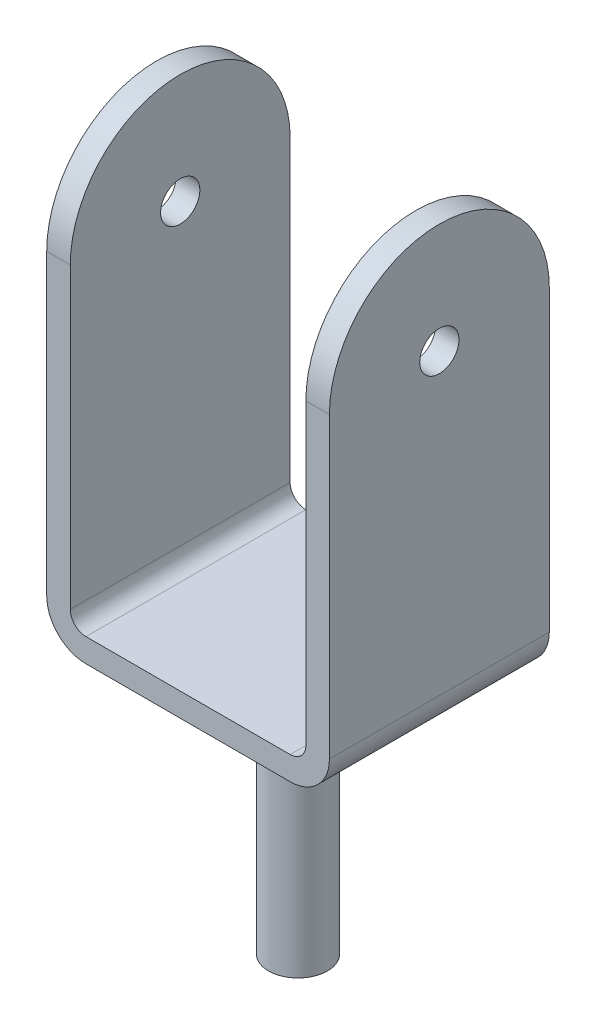
from build123d import *
from build123d.topology import SkipClean

# Parameters (mm, degrees)
BOSS_EXTRUDE1_DEPTH = 280
FILLET1_R           = 50
BOSS_EXTRUDE3_START = -30
BOSS_EXTRUDE3_DEPTH = 30
CUT_EXTRUDE5_START  = -30
CUT_EXTRUDE5_DEPTH  = 30
BOSS_EXTRUDE4_DEPTH = 30
CUT_EXTRUDE6_DEPTH  = 30
BOSS_EXTRUDE5_DEPTH = 325
CUT_EXTRUDE7_REACH  = 708.824
SKETCH7_R           = 25


with BuildPart() as part:
    # Sketch1 → Boss-Extrude1 (new body)
    with BuildSketch(Plane.XY):
        with BuildLine():
            Line((130, 0), (-130, 0))
            ThreePointArc((-130, 0), (-144.142135624, 5.857864376), (-150, 20))
            Line((-150, 20), (-150, 490))
            Line((-150, 490), (-180, 490))
            Line((-180, 490), (-180, -30))
            Line((-180, -30), (180, -30))
            Line((180, -30), (180, 490))
            Line((180, 490), (150, 490))
            Line((150, 490), (150, 20))
            ThreePointArc((150, 20), (144.142135624, 5.857864376), (130, 0))
        make_face()
    extrude(amount=BOSS_EXTRUDE1_DEPTH)

    # Fillet1
    fillet1_edges = [part.edges().sort_by_distance(p)[0] for p in [
        (180, -30, 140),
        (-180, -30, 140),
    ]]
    fillet(fillet1_edges, radius=FILLET1_R)

    # Sketch4 → Boss-Extrude3 (add)
    with BuildSketch(Plane.ZY.offset(180).offset(BOSS_EXTRUDE3_START)):
        with BuildLine():
            Line((247.238052948, 490), (140, 490))
            Line((140, 490), (140, 400))
            Line((140, 400), (280, 400))
            ThreePointArc((280, 400), (271.554793551, 447.888790898), (247.238052948, 490))
        make_face()
        with BuildLine():
            Line((140, 400), (140, 490))
            Line((140, 490), (32.761947052, 490))
            ThreePointArc((32.761947052, 490), (8.445206449, 447.888790898), (0, 400))
            Line((0, 400), (140, 400))
        make_face()
        with BuildLine():
            Line((247.238052948, 490), (140, 490))
            Line((140, 490), (140, 400))
            Line((140, 400), (280, 400))
            ThreePointArc((280, 400), (271.554793551, 447.888790898), (247.238052948, 490))
        make_face()
        with BuildLine():
            Line((140, 400), (140, 490))
            Line((140, 490), (32.761947052, 490))
            ThreePointArc((32.761947052, 490), (8.445206449, 447.888790898), (0, 400))
            Line((0, 400), (140, 400))
        make_face()
        with BuildLine():
            Line((32.761947052, 490), (140, 490))
            Line((140, 490), (247.238052948, 490))
            ThreePointArc((247.238052948, 490), (140, 540), (32.761947052, 490))
        make_face()
    extrude(amount=BOSS_EXTRUDE3_DEPTH)

    # Sketch4<3> → Cut-Extrude5 (cut)
    with SkipClean():  # the faces are left unmerged after this step: merging them gives an invalid solid
        with BuildSketch(Plane.ZY.offset(180).offset(CUT_EXTRUDE5_START)):
            with BuildLine():
                Line((0, 490), (0, 400))
                ThreePointArc((0, 400), (8.445206449, 447.888790898), (32.761947052, 490))
                Line((32.761947052, 490), (0, 490))
            make_face()
            with BuildLine():
                ThreePointArc((247.238052948, 490), (271.554793551, 447.888790898), (280, 400))
                Line((280, 400), (280, 490))
                Line((280, 490), (247.238052948, 490))
            make_face()
        extrude(amount=CUT_EXTRUDE5_DEPTH, mode=Mode.SUBTRACT)

    # Sketch5 → Boss-Extrude4 (add)
    with SkipClean():  # the faces are left unmerged after this step: merging them gives an invalid solid
        with BuildSketch(Plane(origin=(180, 0, 0), x_dir=(0, 0, -1), z_dir=(1, 0, 0))):
            with BuildLine():
                Line((-280, 400), (0, 400))
                ThreePointArc((0, 400), (-140, 540), (-280, 400))
            make_face()
        extrude(amount=-BOSS_EXTRUDE4_DEPTH)

    # Sketch5<2> → Cut-Extrude6 (cut)
    with SkipClean():  # the faces are left unmerged after this step: merging them gives an invalid solid
        with BuildSketch(Plane(origin=(180, 0, 0), x_dir=(0, 0, -1), z_dir=(1, 0, 0))):
            with BuildLine():
                Line((-280, 490), (-280, 400))
                ThreePointArc((-280, 400), (-271.554793551, 447.888790898), (-247.238052948, 490))
                Line((-247.238052948, 490), (-280, 490))
            make_face()
            with BuildLine():
                ThreePointArc((-32.761947052, 490), (-8.445206449, 447.888790898), (0, 400))
                Line((0, 400), (0, 490))
                Line((0, 490), (-32.761947052, 490))
            make_face()
        extrude(amount=-CUT_EXTRUDE6_DEPTH, mode=Mode.SUBTRACT)

    # Sketch6 → Boss-Extrude5 (add)
    with SkipClean():  # the faces are left unmerged after this step: merging them gives an invalid solid
        with BuildSketch(Plane.XZ.offset(30)):
            with BuildLine():
                ThreePointArc((37.5, 140), (26.516504294, 166.516504294), (0, 177.5))
                Line((0, 177.5), (0, 102.5))
                ThreePointArc((0, 102.5), (26.516504294, 113.483495706), (37.5, 140))
            make_face()
            with BuildLine():
                Line((0, 102.5), (0, 177.5))
                ThreePointArc((0, 177.5), (-37.5, 140), (0, 102.5))
            make_face()
            with BuildLine():
                ThreePointArc((37.5, 140), (26.516504294, 166.516504294), (0, 177.5))
                Line((0, 177.5), (0, 102.5))
                ThreePointArc((0, 102.5), (26.516504294, 113.483495706), (37.5, 140))
            make_face()
            with BuildLine():
                Line((0, 102.5), (0, 177.5))
                ThreePointArc((0, 177.5), (-37.5, 140), (0, 102.5))
            make_face()
        extrude(amount=BOSS_EXTRUDE5_DEPTH)

    # Cut-Extrude7: up to this face of the body (flat: up to its plane)
    cut_extrude7_end = Plane(part.part.faces().sort_by_distance((180, 210, 140))[0])
    # Sketch7 → Cut-Extrude7 (cut, up to the picked face)
    with BuildSketch(Plane.ZY.offset(180), mode=Mode.PRIVATE) as cut_extrude7_sk1:
        with Locations(Location((140, 400, 0), (0, 0, 270))):
            Circle(SKETCH7_R)
    cut_extrude7_tool1 = split(extrude(cut_extrude7_sk1.sketch, amount=-CUT_EXTRUDE7_REACH, mode=Mode.PRIVATE), bisect_by=cut_extrude7_end, keep=Keep.BOTH, mode=Mode.PRIVATE)
    add(cut_extrude7_tool1.solids().sort_by(Axis((-180, 400, 140), (1, 0, 0)))[0], mode=Mode.SUBTRACT)


solid = part.part
